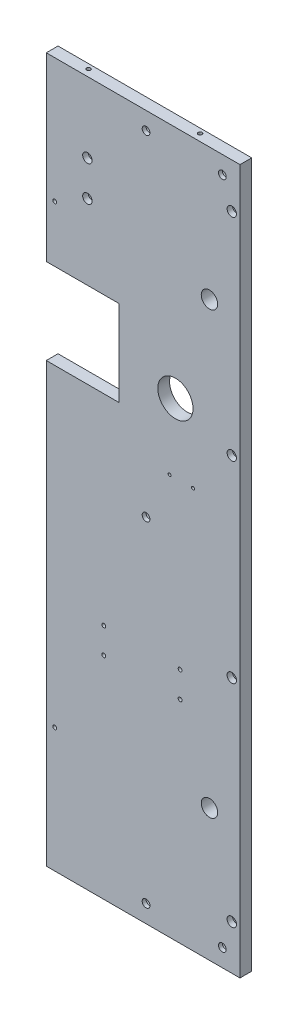
from build123d import *

# Parameters (mm, degrees)
SKETCH_1_W                  = 165
SKETCH_1_H                  = 600
EXTRUDE_1_DEPTH             = 10
SKETCH_5_R                  = 15
CUT_EXTRUDE_1_DEPTH         = 322.442063209
HOLE_WIZARD_M4_1_D          = 3.3
HOLE_WIZARD_M3_1_D          = 2.5
HOLE_WIZARD_M4_3_D          = 3.3
SKETCH_18_R                 = 7
CUT_EXTRUDE_2_DEPTH         = 322.442063209
HOLE_WIZARD_M4_4_D          = 3.3
HOLE_WIZARD_M4_4_DEPTH      = 10
HOLE_WIZARD_M4_4_TIP        = 0.991420021
HOLE_WIZARD_M4_5_D          = 3.3
HOLE_WIZARD_M4_5_DEPTH      = 10.1
HOLE_WIZARD_M4_5_TIP        = 0.991420021
HOLE_WIZARD_6_D             = 4.5
HOLE_WIZARD_6_CBORE_D       = 8
HOLE_WIZARD_6_CBORE_DEPTH   = 4.6
SKETCH_27_W                 = 71.16849895
SKETCH_27_H                 = 73
CUT_EXTRUDE_3_DEPTH         = 322.442063209
HOLE_WIZARD_5_D             = 4.5
HOLE_WIZARD_5_CBORE_D       = 8
HOLE_WIZARD_5_CBORE_DEPTH   = 4.6
HOLE_WIZARD_6_2_D           = 6.6
HOLE_WIZARD_6_2_CBORE_D     = 11
HOLE_WIZARD_6_2_CBORE_DEPTH = 6.8


with BuildPart() as part:
    # 草图1 → 凸台-拉伸1 (new body)
    with BuildSketch(Plane.XY):
        with Locations((-32.5, 0)):
            Rectangle(SKETCH_1_W, SKETCH_1_H)
    extrude(amount=EXTRUDE_1_DEPTH)

    # 草图5 → 切除-拉伸1 (cut, through all)
    with BuildSketch(Plane.XY.offset(10)):
        with Locations((-5, 100)):
            Circle(SKETCH_5_R)
    extrude(amount=-CUT_EXTRUDE_1_DEPTH, mode=Mode.SUBTRACT)

    # M4 螺纹孔1 (through all)
    with Locations(Plane.XY.offset(10)):
        with Locations((-66, -120), (-1, -98), (-1, -120), (-66, -98)):
            Hole(HOLE_WIZARD_M4_1_D / 2)

    # M3 螺纹孔1 (through all)
    with Locations(Plane.XY.offset(10)):
        with Locations((-10, 41.3), (10, 41.3)):
            Hole(HOLE_WIZARD_M3_1_D / 2)

    # M4 螺纹孔3 (through all)
    with Locations(Plane(origin=(0, 0, 0), x_dir=(-1, 0, 0), z_dir=(0, 0, -1))):
        with Locations((107.75, 193.999999998), (107.75, -194.000000002)):
            Hole(HOLE_WIZARD_M4_3_D / 2)

    # 草图18 → 切除-拉伸2 (cut, through all)
    with BuildSketch(Plane(origin=(0, 0, 0), x_dir=(-1, 0, 0), z_dir=(0, 0, -1))):
        with Locations((-24, 187.5)):
            Circle(SKETCH_18_R)
        with Locations((-24, -187.5)):
            Circle(SKETCH_18_R)
    extrude(amount=-CUT_EXTRUDE_2_DEPTH, mode=Mode.SUBTRACT)

    # M4 螺纹孔4
    with Locations(Plane(origin=(0, -300, 0), x_dir=(-1, 0, 0), z_dir=(0, -1, 0))):
        with Locations((-10, -4), (85, -4)):
            Hole(HOLE_WIZARD_M4_4_D / 2, depth=HOLE_WIZARD_M4_4_DEPTH)
            with Locations((0, 0, -(HOLE_WIZARD_M4_4_DEPTH + HOLE_WIZARD_M4_4_TIP / 2))):  # 118° drill point
                Cone(0, HOLE_WIZARD_M4_4_D / 2, HOLE_WIZARD_M4_4_TIP, mode=Mode.SUBTRACT)

    # M4 螺纹孔5
    with Locations(Plane(origin=(0, 300, 0), x_dir=(1, 0, 0), z_dir=(0, 1, 0))):
        with Locations((-85, -4), (10, -4)):
            Hole(HOLE_WIZARD_M4_5_D / 2, depth=HOLE_WIZARD_M4_5_DEPTH)
            with Locations((0, 0, -(HOLE_WIZARD_M4_5_DEPTH + HOLE_WIZARD_M4_5_TIP / 2))):  # 118° drill point
                Cone(0, HOLE_WIZARD_M4_5_D / 2, HOLE_WIZARD_M4_5_TIP, mode=Mode.SUBTRACT)

    # Hole Wizard 6 (through all)
    with Locations(Plane.XY.offset(10)):
        with Locations((43, 262), (43, 82), (43, -82), (43, -262)):
            CounterBoreHole(HOLE_WIZARD_6_D / 2, HOLE_WIZARD_6_CBORE_D / 2, HOLE_WIZARD_6_CBORE_DEPTH)

    # 草图27 → 切除-拉伸3 (cut, through all)
    with BuildSketch(Plane(origin=(0, 0, 0), x_dir=(-1, 0, 0), z_dir=(0, 0, -1))):
        with Locations((88.584249475, 109.5)):
            Rectangle(SKETCH_27_W, SKETCH_27_H)
    extrude(amount=-CUT_EXTRUDE_3_DEPTH, mode=Mode.SUBTRACT)

    # 打孔尺寸根据内六角圆柱头螺钉的类型5 (through all)
    with Locations(Plane.XY.offset(10)):
        with Locations((-80, 240), (-80, 210)):
            CounterBoreHole(HOLE_WIZARD_5_D / 2, HOLE_WIZARD_5_CBORE_D / 2, HOLE_WIZARD_5_CBORE_DEPTH)

    # Hole Wizard 6 2 (through all)
    with Locations(Plane(origin=(0, 0, 0), x_dir=(-1, 0, 0), z_dir=(0, 0, -1))):
        with Locations((30.000000001, 285), (-35, 285), (30.000000001, 2e-09), (30.000000001, -284.999999998), (-35, -284.999999998)):
            CounterBoreHole(HOLE_WIZARD_6_2_D / 2, HOLE_WIZARD_6_2_CBORE_D / 2, HOLE_WIZARD_6_2_CBORE_DEPTH)


solid = part.part
